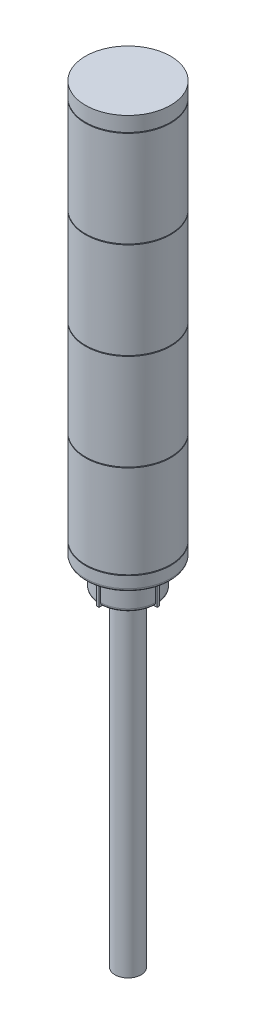
SolidWorks part; units mm, degrees
ref_plane "前视基准面" through (0, 0, 0) normal (0, 0, 1) x (1, 0, 0)
ref_plane "上视基准面" through (0, 0, 0) normal (0, 1, 0) x (1, 0, 0)
ref_plane "右视基准面" through (0, 0, 0) normal (1, 0, 0) x (0, 0, -1)
sketch "草图1" plane through (0, 0, 0) normal (0, 0, 1) x (1, 0, 0)
  line L0 (0, 0) -> (-8, 0)
  line L1 (-8, 0) -> (-8, 200)
  line L2 (-8, 200) -> (-15.5, 200)
  line L3 (-17.5, 202) -> (-17.5, 214)
  line L4 (-19.2217, 215.9805) -> (-24.2783, 216.6912)
  line L5 (-26, 218.6717) -> (-26, 469)
  line L6 (-26, 469) -> (0, 469)
  line L7 (0, 0) -> (0, 469)
  line L8 (0, 0) -> (0, 888.6012) construction
  arc A0 (-17.5, 202) -> (-15.5, 200) centre (-15.5, 202) ccw
  arc A1 (-17.5, 214) -> (-19.2217, 215.9805) centre (-19.5, 214) ccw
  arc A2 (-24.2783, 216.6912) -> (-26, 218.6717) centre (-24, 218.6717) cw
  dimension "D5" = 2
  dimension "D1" = 16
  dimension "D2" = 52
  dimension "D3" = 35
  dimension "D4" = 200
  dimension "D6" = 12
  dimension "D7" = 8
  dimension "L" = 469
revolve "旋转1" add sketch "草图1" angle 360 about L8
sketch "草图2" plane through (0, 0, 0) normal (0, 0, 1) x (1, 0, 0)
  line L0 (-15.5, 200) -> (15.5, 200) construction
  line L1 (23, 226) -> (29, 226)
  line L2 (23, 226) -> (23, 225.5)
  line L3 (23, 225.5) -> (29, 225.5)
  line L4 (29, 226) -> (29, 225.5)
  line L5 (23, 283) -> (29, 283)
  line L6 (23, 283) -> (23, 282.5)
  line L7 (23, 282.5) -> (29, 282.5)
  line L8 (29, 283) -> (29, 282.5)
  line L9 (23, 342) -> (29, 342)
  line L10 (23, 342) -> (23, 341.5)
  line L11 (23, 341.5) -> (29, 341.5)
  line L12 (29, 342) -> (29, 341.5)
  line L13 (23, 401) -> (29, 401)
  line L14 (23, 401) -> (23, 400.5)
  line L15 (23, 400.5) -> (29, 400.5)
  line L16 (29, 401) -> (29, 400.5)
  line L17 (23, 460) -> (29, 460)
  line L18 (23, 460) -> (23, 459.5)
  line L19 (23, 459.5) -> (29, 459.5)
  line L20 (29, 460) -> (29, 459.5)
  line L21 (23, 519) -> (29, 519)
  line L22 (23, 519) -> (23, 518.5)
  line L23 (23, 518.5) -> (29, 518.5)
  line L24 (29, 519) -> (29, 518.5)
  line L25 (23, 578) -> (29, 578)
  line L26 (23, 578) -> (23, 577.5)
  line L27 (23, 577.5) -> (29, 577.5)
  line L28 (29, 578) -> (29, 577.5)
  line L29 (8, 0) -> (8, 200) construction
  dimension "D1" = 26
  dimension "D2" = 15
  dimension "D3" = 6
  dimension "D4" = 0.5
  dimension "D5" = 57
  dimension "D6" = 59
  dimension "D7" = 59
  dimension "D8" = 59
  dimension "D9" = 59
  dimension "D10" = 59
  dimension "D11" = 0.5
  dimension "D12" = 0.5
  dimension "D13" = 0.5
  dimension "D14" = 0.5
  dimension "D15" = 0.5
  dimension "D16" = 0.5
ref_axis "基准轴1" through (0, 616.35, 0) along (0, -1, 0)
revolve "切除-旋转1" cut sketch "草图2" angle 360 about axis through (0, 616.35, 0) along (0, -1, 0)
sketch "草图3" plane through (0, 200, 0) normal (0, -1, 0) x (1, 0, 0)
  line L0 (18.5, -0.75) -> (12.5, -0.75)
  line L1 (-0.75, 18.5) -> (0.75, 18.5)
  line L2 (-0.75, 18.5) -> (-0.75, 12.5)
  line L3 (-0.75, 12.5) -> (0.75, 12.5)
  line L4 (0.75, 18.5) -> (0.75, 12.5)
  line L5 (-0.75, 18.5) -> (0.75, 12.5) construction
  line L6 (-0.75, 12.5) -> (0.75, 18.5) construction
  line L7 (18.5, 0.75) -> (12.5, 0.75)
  line L8 (18.5, 0.75) -> (18.5, -0.75)
  line L9 (12.5, 0.75) -> (12.5, -0.75)
  line L10 (-0.75, -18.5) -> (-0.75, -12.5)
  line L11 (0.75, -18.5) -> (0.75, -12.5)
  line L12 (0.75, -18.5) -> (-0.75, -18.5)
  line L13 (0.75, -12.5) -> (-0.75, -12.5)
  line L14 (-18.5, 0.75) -> (-12.5, 0.75)
  line L15 (-18.5, -0.75) -> (-12.5, -0.75)
  line L16 (-18.5, -0.75) -> (-18.5, 0.75)
  line L17 (-12.5, -0.75) -> (-12.5, 0.75)
  circle A0 centre (0, 0) radius 15.5 construction
  point P0 (0, 15.5)
  point P7 (-12.5, 0)
  point P9 (12.5, 0)
  dimension "D1" = 6
  dimension "D2" = 1.5
  dimension "D3" = 4
extrude "凸台-拉伸1" add sketch "草图3" against normal up to next
